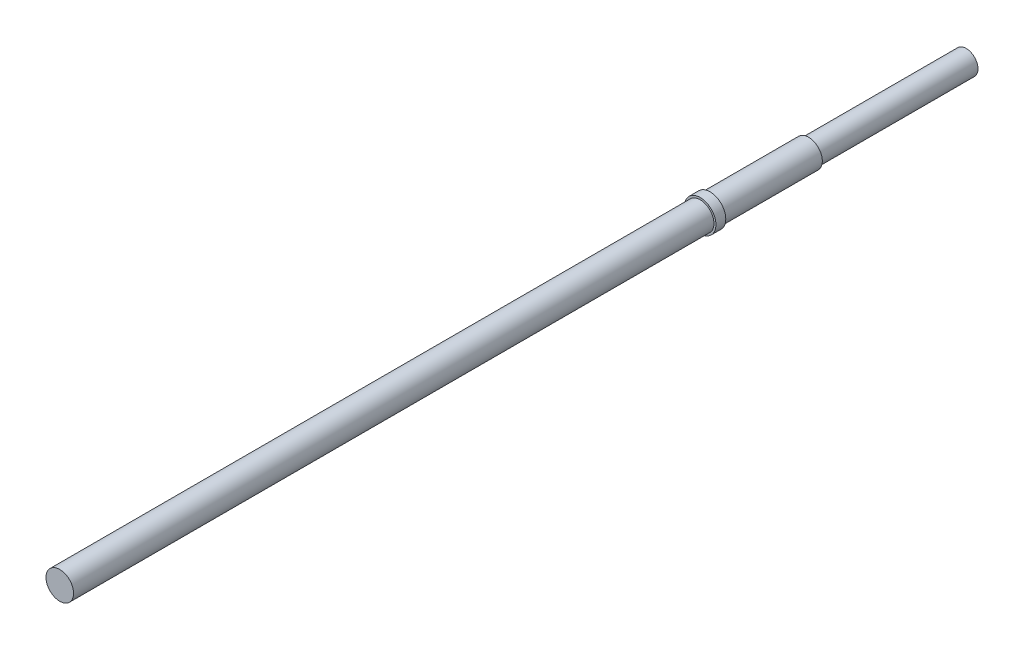
SolidWorks part; units mm, degrees
ref_plane "前视基准面" through (0, 0, 0) normal (0, 0, 1) x (1, 0, 0)
ref_plane "上视基准面" through (0, 0, 0) normal (0, 1, 0) x (1, 0, 0)
ref_plane "右视基准面" through (0, 0, 0) normal (1, 0, 0) x (0, 0, -1)
sketch "草图1" plane through (0, 0, 0) normal (0, 0, 1) x (1, 0, 0)
  circle A0 centre (0, 0) radius 6
  dimension "D1" = 12
extrude "凸台-拉伸1" add sketch "草图1" along normal blind 80
sketch "草图3" plane through (0, 0, 80) normal (0, 0, 1) x (1, 0, 0)
  circle A0 centre (0, 0) radius 7
  dimension "D1" = 14
extrude "凸台-拉伸2" add sketch "草图3" along normal blind 380
sketch "草图4" plane through (0, 0, 460) normal (0, 0, 1) x (1, 0, 0)
  circle A0 centre (0, 0) radius 8
  dimension "D1" = 16
extrude "凸台-拉伸3" add sketch "草图4" along normal blind 5 from offset 330
